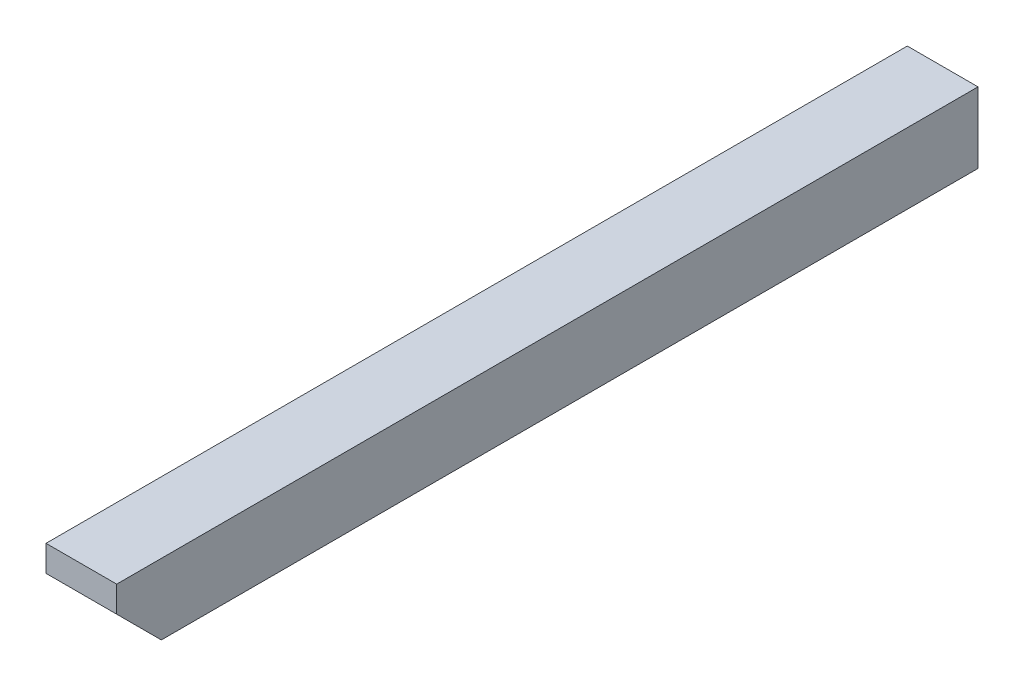
from build123d import *

# Parameters (mm, degrees)
SKETCH1_W           = 19
SKETCH1_H           = 19
BOSS_EXTRUDE1_DEPTH = 115.75
CHAMFER1_SIZE       = 12


with BuildPart() as part:
    # Sketch1 → Boss-Extrude1 (new, symmetric)
    with BuildSketch(Plane.XY):
        Rectangle(SKETCH1_W, SKETCH1_H)
    extrude(amount=BOSS_EXTRUDE1_DEPTH, both=True)

    # Chamfer1
    chamfer1_edges = [part.edges().sort_by_distance(p)[0] for p in [
        (0, -9.5, 115.75),
    ]]
    chamfer(chamfer1_edges, length=CHAMFER1_SIZE)


solid = part.part
